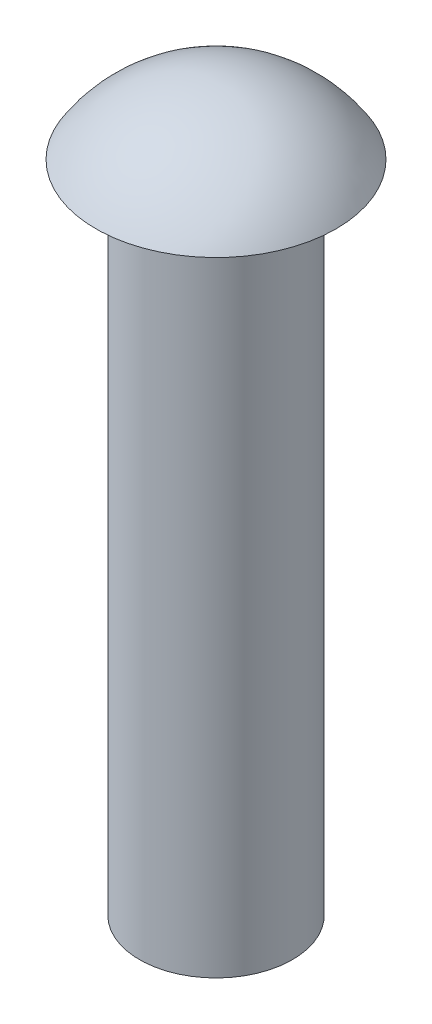
SolidWorks part; units mm, degrees
ref_plane "前视基准面" through (0, 0, 0) normal (0, 0, 1) x (1, 0, 0)
ref_plane "上视基准面" through (0, 0, 0) normal (0, 1, 0) x (1, 0, 0)
ref_plane "右视基准面" through (0, 0, 0) normal (1, 0, 0) x (0, 0, -1)
sketch "草图1" plane through (0, 0, 0) normal (0, 0, 1) x (1, 0, 0)
  line L0 (0, -15) -> (0, 15)
  line L2 (3.5, 14.9613) -> (3.5, -15)
  line L3 (3.5, -15) -> (0, -15)
  line L4 (0, 15) -> (0, 18)
  line L5 (3.5, 14.9613) -> (5.5, 14.9613)
  arc A0 (0, 18) -> (5.5, 14.9613) centre (0, 11.5032) cw
  point P4 (0, 0)
  dimension "D1" = 30
  dimension "D2" = 3.5
  dimension "D3" = 3
  dimension "D4" = 2
revolve "旋转1" add sketch "草图1" angle 360 about L0
